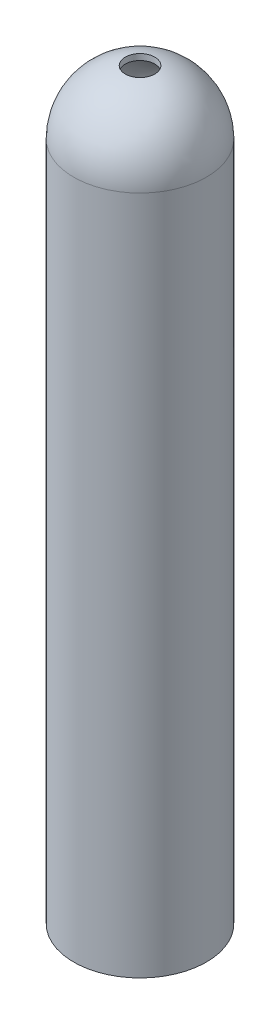
from build123d import *


with BuildPart() as part:
    # Sketch1 → Revolve1 (revolve)
    with BuildSketch(Plane.XY, mode=Mode.PRIVATE) as revolve1_sk:
        with BuildLine():
            Line((-2.25, 0), (-2.25, 23.046514453))
            ThreePointArc((-2.25, 23.046514453), (-1.757337108, 24.433958146), (-0.5, 25.2))
            Line((-0.5, 25.2), (-0.5, 24.99523198))
            ThreePointArc((-0.5, 24.99523198), (-1.615247584, 24.291504413), (-2.05, 23.046514453))
            Line((-2.05, 23.046514453), (-2.05, 0))
            Line((-2.05, 0), (-2.25, 0))
        make_face()
    revolve(revolve1_sk.sketch.rotate(Axis((0, 0, 0), (0, 1, 0)), 270), axis=Axis((0, 0, 0), (0, 1, 0)))


solid = part.part
